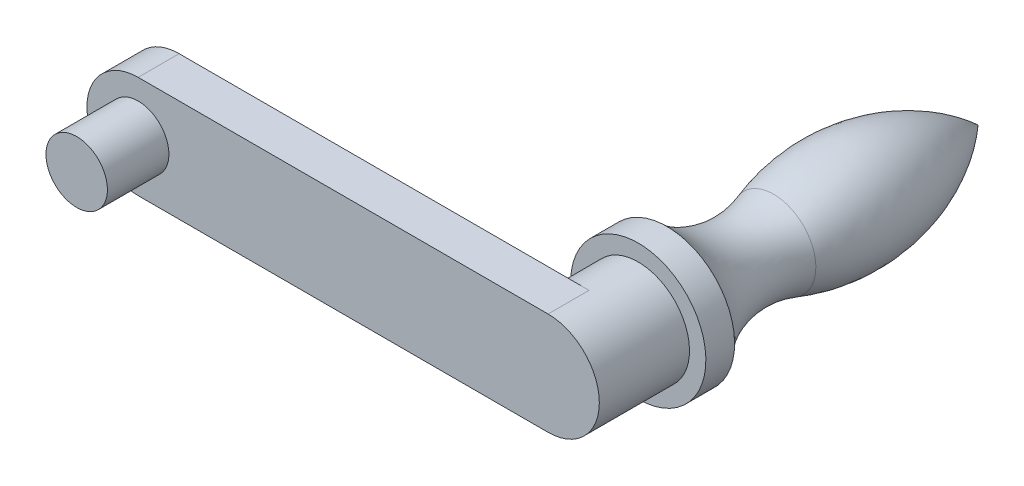
SolidWorks part; units mm, degrees
ref_plane "前视基准面" through (0, 0, 0) normal (0, 0, 1) x (1, 0, 0)
ref_plane "上视基准面" through (0, 0, 0) normal (0, 1, 0) x (1, 0, 0)
ref_plane "右视基准面" through (0, 0, 0) normal (1, 0, 0) x (0, 0, -1)
sketch "草图1" plane through (0, 0, 0) normal (0, 0, 1) x (1, 0, 0)
  line L1 (0, 0) -> (100, 0)
  line L3 (0, 25) -> (100, 25)
  arc A0 (0, 25) -> (0, 0) centre (0, 12.5) ccw
  arc A1 (100, 0) -> (100, 25) centre (100, 12.5) ccw
extrude "凸台-拉伸1" add sketch "草图1" along normal blind 10
sketch "草图2" plane through (0, 0, 10) normal (0, 0, 1) x (1, 0, 0)
  circle A0 centre (0, 12.5) radius 7.5
extrude "凸台-拉伸2" add sketch "草图2" along normal blind 15
sketch "草图3" plane through (0, 0, 0) normal (0, 0, -1) x (-1, 0, 0)
  circle A0 centre (-100, 12.5) radius 12.5
ref_plane "基准面1" through (100, 0, 0) normal (1, 0, 0) x (0, 0, -1)
sketch "草图7" plane through (100, 0, 0) normal (1, 0, 0) x (0, 0, -1)
  line L0 (0, 12.5) -> (94.8859, 12.5) construction
  line L1 (0, 0) -> (0, 25) construction
  line L2 (0, 12.5) -> (0, 25)
  line L3 (0, 25) -> (12, 25)
  line L4 (12, 25) -> (12, 29)
  line L5 (12, 29) -> (19, 29)
  line L6 (0, 12.5) -> (94.8859, 12.5)
  arc A0 (19, 29) -> (45.0326, 22.795) centre (36.9165, 46.4559) ccw
  arc A2 (45.0326, 22.795) -> (94.8859, 12.5) centre (61.2556, -24.5) cw
  dimension "D1" = 37
  dimension "D4" = 50
  dimension "D2" = 12
  dimension "D5" = 7
revolve "旋转1" add sketch "草图7" angle 360 about L6
